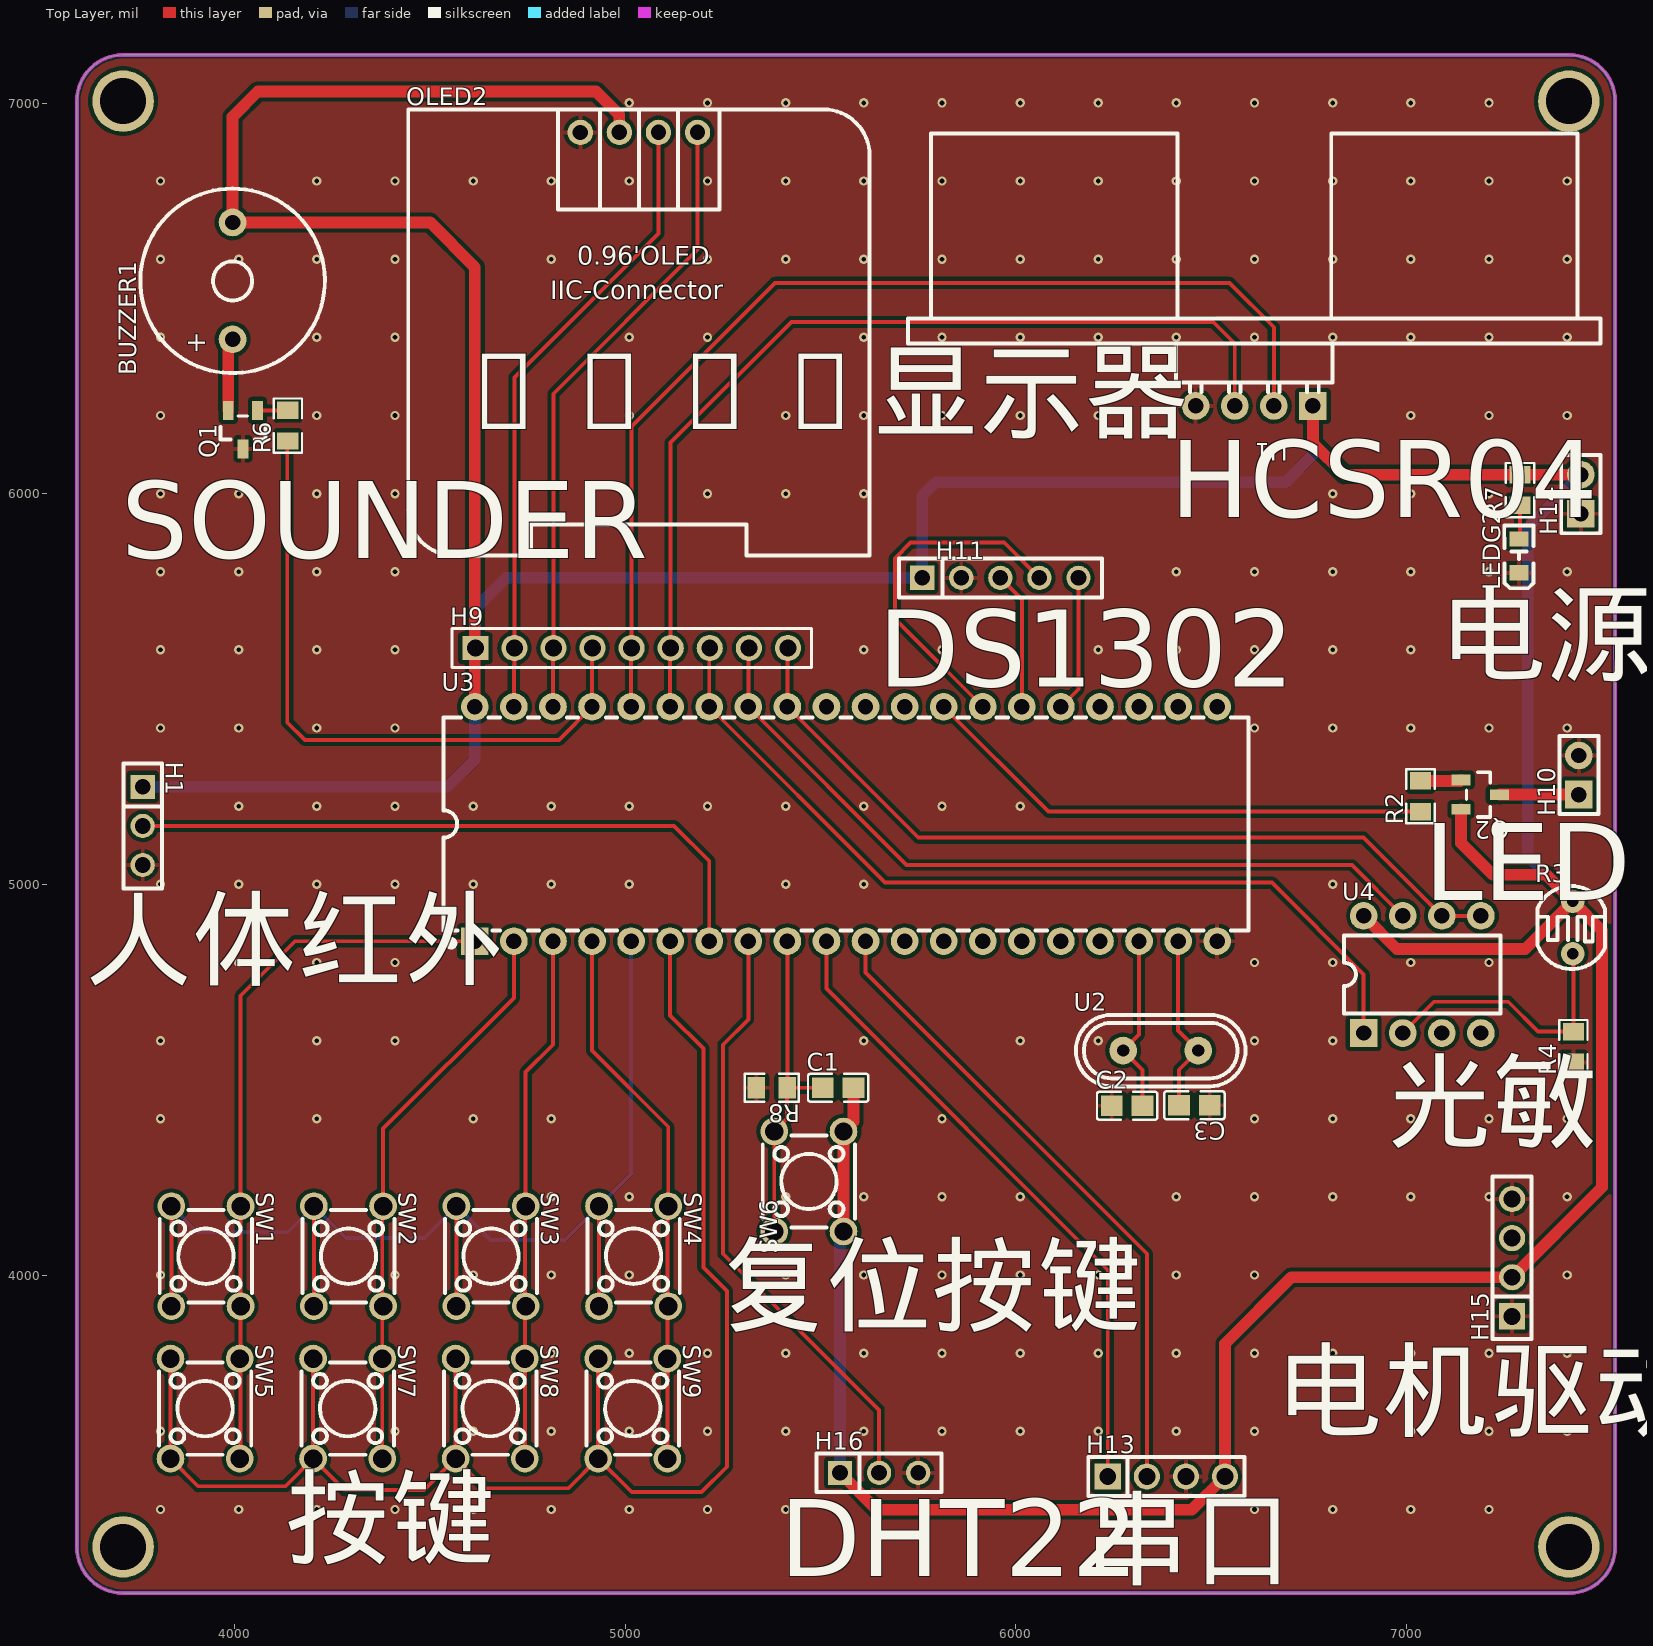
[diagram p0: Top Layer view]
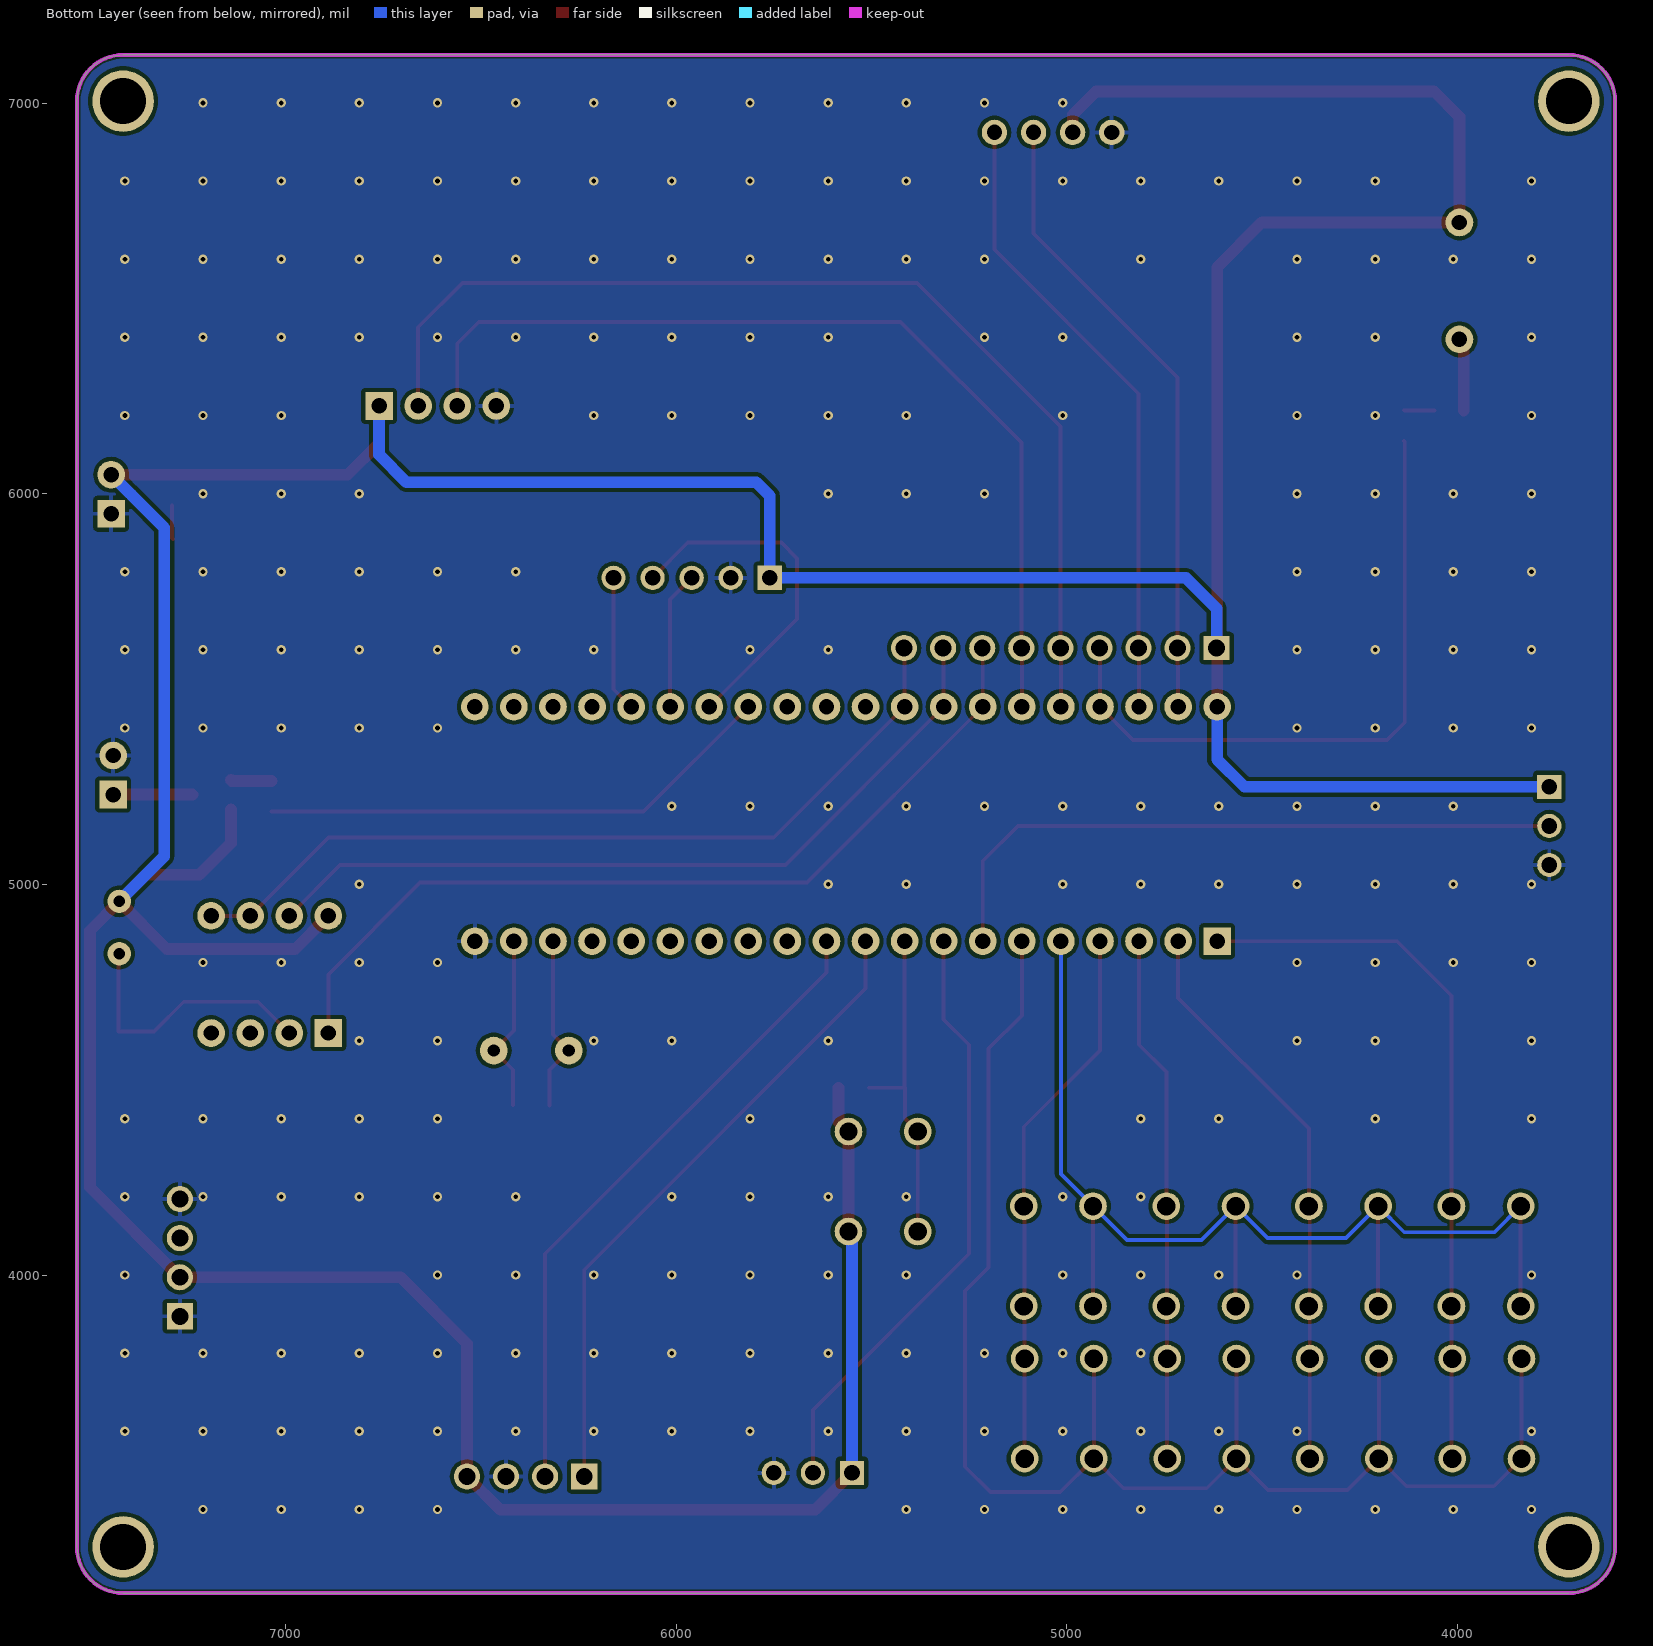
[diagram p1: Bottom Layer view, seen from below]
# Altium PCB MISC52077.pcbdoc
Units mil, origin at the board's own origin, x right, y up, seen from the top; angles counter-clockwise.
Board outline 3937.01 x 3937.01 mil, 2 copper layers (Top Layer, Bottom Layer), stack 62.206 mil thick; 35 components, 34 nets, 158 pads, 232 vias.

## Layer stack, top to bottom
Top Solder Mask Layer: solder mask 0.394, Dk 3.3
Top Layer: signal copper 1.379
Dielectric1: surface 59.449, FR4, Dk 4.5
Bottom Layer: signal copper 1.378
Bottom Solder Mask Layer: solder mask 0.394, Dk 3.3

## Board outline
3596.5,3304.61 ccw(c3714.61,3304.61) 3714.61,3186.5 7415.39,3186.5 ccw(c7415.39,3304.61) 7533.5,3304.61 7533.5,7005.39 ccw(c7415.39,7005.39) 7415.39,7123.5 3714.61,7123.5 ccw(c3714.61,7005.39) 3596.5,7005.39

## Design rules (kind name [scope] priority, off if disabled: settings)
BoardOutlineClearance copperThickness2oz_1 [All] p2 off: genericclearance=7.99 ignorepadtopadclearanceinfootprint=FALSE except(0: Arc-SplitContinuation Track-SplitContinuation SMDPad-SplitContinuation THPad-SplitContinuation Via-SplitContinuation Fill-SplitContinuation Region-SplitContinuation Poly-SplitContinuation Text-SplitContinuation Hole-SplitContinuation; 5.98: Arc-CutoutEdge Track-CutoutEdge SMDPad-CutoutEdge THPad-CutoutEdge Via-CutoutEdge Text-CutoutEdge; 6.9: Hole-OutlineEdge Hole-CutoutEdge; 10: Poly-OutlineEdge Poly-CutoutEdge; 11.81: Arc-OutlineEdge Track-OutlineEdge SMDPad-OutlineEdge THPad-OutlineEdge Via-OutlineEdge Fill-OutlineEdge Region-OutlineEdge Text-OutlineEdge Fill-CutoutEdge Region-CutoutEdge)
BoardOutlineClearance Plane_innerPlane_1 [All] p4 off: genericclearance=4.02 ignorepadtopadclearanceinfootprint=FALSE except(0: Arc-SplitContinuation Track-SplitContinuation SMDPad-SplitContinuation THPad-SplitContinuation Via-SplitContinuation Fill-SplitContinuation Region-SplitContinuation Poly-SplitContinuation Text-SplitContinuation Hole-SplitContinuation; 5.98: Arc-CutoutEdge Track-CutoutEdge SMDPad-CutoutEdge THPad-CutoutEdge Via-CutoutEdge Text-CutoutEdge; 6.9: Hole-OutlineEdge Hole-CutoutEdge; 10: Poly-OutlineEdge Poly-CutoutEdge; 11.81: Arc-OutlineEdge Track-OutlineEdge SMDPad-OutlineEdge THPad-OutlineEdge Via-OutlineEdge Fill-OutlineEdge Region-OutlineEdge Text-OutlineEdge Fill-CutoutEdge Region-CutoutEdge)
BoardOutlineClearance Copper_copperRegion_1 [All] p6 off: genericclearance=4.02 ignorepadtopadclearanceinfootprint=FALSE except(0: Arc-SplitContinuation Track-SplitContinuation SMDPad-SplitContinuation THPad-SplitContinuation Via-SplitContinuation Fill-SplitContinuation Region-SplitContinuation Poly-SplitContinuation Text-SplitContinuation Hole-SplitContinuation; 5.98: Arc-CutoutEdge Track-CutoutEdge SMDPad-CutoutEdge THPad-CutoutEdge Via-CutoutEdge Text-CutoutEdge; 6.9: Hole-OutlineEdge Hole-CutoutEdge; 10: Poly-OutlineEdge Poly-CutoutEdge; 11.81: Arc-OutlineEdge Track-OutlineEdge SMDPad-OutlineEdge THPad-OutlineEdge Via-OutlineEdge Fill-OutlineEdge Region-OutlineEdge Text-OutlineEdge Fill-CutoutEdge Region-CutoutEdge)
BoardOutlineClearance Copper_copperRegion_copperThickness1oz_1 [All] p8 off: genericclearance=4.02 ignorepadtopadclearanceinfootprint=FALSE except(0: Arc-SplitContinuation Track-SplitContinuation SMDPad-SplitContinuation THPad-SplitContinuation Via-SplitContinuation Fill-SplitContinuation Region-SplitContinuation Poly-SplitContinuation Text-SplitContinuation Hole-SplitContinuation; 5.98: Arc-CutoutEdge Track-CutoutEdge SMDPad-CutoutEdge THPad-CutoutEdge Via-CutoutEdge Text-CutoutEdge; 6.9: Hole-OutlineEdge Hole-CutoutEdge; 10: Poly-OutlineEdge Poly-CutoutEdge; 11.81: Arc-OutlineEdge Track-OutlineEdge SMDPad-OutlineEdge THPad-OutlineEdge Via-OutlineEdge Fill-OutlineEdge Region-OutlineEdge Text-OutlineEdge Fill-CutoutEdge Region-CutoutEdge)
BoardOutlineClearance Copper_copperRegion_Copper_copperRegion_1 [All] p10 off: genericclearance=4.02 ignorepadtopadclearanceinfootprint=FALSE except(0: Arc-SplitContinuation Track-SplitContinuation SMDPad-SplitContinuation THPad-SplitContinuation Via-SplitContinuation Fill-SplitContinuation Region-SplitContinuation Poly-SplitContinuation Text-SplitContinuation Hole-SplitContinuation; 5.98: Arc-CutoutEdge Track-CutoutEdge SMDPad-CutoutEdge THPad-CutoutEdge Via-CutoutEdge Text-CutoutEdge; 6.9: Hole-OutlineEdge Hole-CutoutEdge; 10: Poly-OutlineEdge Poly-CutoutEdge; 11.81: Arc-OutlineEdge Track-OutlineEdge SMDPad-OutlineEdge THPad-OutlineEdge Via-OutlineEdge Fill-OutlineEdge Region-OutlineEdge Text-OutlineEdge Fill-CutoutEdge Region-CutoutEdge)
BoardOutlineClearance copperThickness1oz_1 [All] p12: genericclearance=4.02 ignorepadtopadclearanceinfootprint=FALSE except(0: Arc-SplitContinuation Track-SplitContinuation SMDPad-SplitContinuation THPad-SplitContinuation Via-SplitContinuation Fill-SplitContinuation Region-SplitContinuation Poly-SplitContinuation Text-SplitContinuation Hole-SplitContinuation; 5.98: Arc-CutoutEdge Track-CutoutEdge SMDPad-CutoutEdge THPad-CutoutEdge Via-CutoutEdge Text-CutoutEdge; 6.9: Hole-OutlineEdge Hole-CutoutEdge; 10: Poly-OutlineEdge Poly-CutoutEdge; 11.81: Arc-OutlineEdge Track-OutlineEdge SMDPad-OutlineEdge THPad-OutlineEdge Via-OutlineEdge Fill-OutlineEdge Region-OutlineEdge Text-OutlineEdge Fill-CutoutEdge Region-CutoutEdge)
Clearance copperThickness2oz [All] p1 off: gap=7.99 ignorepadtopadclearanceinfootprint=FALSE except(5.98: SMDPad-Track SMDPad-SMDPad THPad-Track SMDPad-THPad THPad-THPad Track-Via SMDPad-Via THPad-Via Via-Via Fill-SMDPad Region-SMDPad Fill-THPad Region-THPad Fill-Via Region-Via Fill-Fill Fill-Region Region-Region Arc-Track Arc-SMDPad Arc-THPad Arc-Via Fill-Arc Region-Arc Arc-Arc Text-Track SMDPad-Text Text-THPad Text-Via Fill-Text Region-Text Arc-Text Text-Text; 6.9: Hole-Track Hole-SMDPad Hole-THPad Hole-Via Fill-Hole Region-Hole Hole-Arc Hole-Text; 10: Poly-Track Poly-SMDPad Poly-THPad Poly-Via Poly-Fill Poly-Region Poly-Poly Poly-Arc Poly-Text Poly-Hole; 11.81: Fill-Track Region-Track)
Clearance Plane_innerPlane [All] p3 off: gap=4.02 ignorepadtopadclearanceinfootprint=FALSE except(5.98: SMDPad-Track SMDPad-SMDPad THPad-Track SMDPad-THPad THPad-THPad Track-Via SMDPad-Via THPad-Via Via-Via Fill-SMDPad Region-SMDPad Fill-THPad Region-THPad Fill-Via Region-Via Fill-Fill Fill-Region Region-Region Arc-Track Arc-SMDPad Arc-THPad Arc-Via Fill-Arc Region-Arc Arc-Arc Text-Track SMDPad-Text Text-THPad Text-Via Fill-Text Region-Text Arc-Text Text-Text; 6.9: Hole-Track Hole-SMDPad Hole-THPad Hole-Via Fill-Hole Region-Hole Hole-Arc Hole-Text; 10: Poly-Track Poly-SMDPad Poly-THPad Poly-Via Poly-Fill Poly-Region Poly-Poly Poly-Arc Poly-Text Poly-Hole; 11.81: Fill-Track Region-Track)
Clearance Copper_copperRegion [All] p5 off: gap=4.02 ignorepadtopadclearanceinfootprint=FALSE except(5.98: SMDPad-Track SMDPad-SMDPad THPad-Track SMDPad-THPad THPad-THPad Track-Via SMDPad-Via THPad-Via Via-Via Fill-SMDPad Region-SMDPad Fill-THPad Region-THPad Fill-Via Region-Via Fill-Fill Fill-Region Region-Region Arc-Track Arc-SMDPad Arc-THPad Arc-Via Fill-Arc Region-Arc Arc-Arc Text-Track SMDPad-Text Text-THPad Text-Via Fill-Text Region-Text Arc-Text Text-Text; 6.9: Hole-Track Hole-SMDPad Hole-THPad Hole-Via Fill-Hole Region-Hole Hole-Arc Hole-Text; 10: Poly-Track Poly-SMDPad Poly-THPad Poly-Via Poly-Fill Poly-Region Poly-Poly Poly-Arc Poly-Text Poly-Hole; 11.81: Fill-Track Region-Track)
Clearance Copper_copperRegion_copperThickness1oz [All] p7 off: gap=4.02 ignorepadtopadclearanceinfootprint=FALSE except(5.98: SMDPad-Track SMDPad-SMDPad THPad-Track SMDPad-THPad THPad-THPad Track-Via SMDPad-Via THPad-Via Via-Via Fill-SMDPad Region-SMDPad Fill-THPad Region-THPad Fill-Via Region-Via Fill-Fill Fill-Region Region-Region Arc-Track Arc-SMDPad Arc-THPad Arc-Via Fill-Arc Region-Arc Arc-Arc Text-Track SMDPad-Text Text-THPad Text-Via Fill-Text Region-Text Arc-Text Text-Text; 6.9: Hole-Track Hole-SMDPad Hole-THPad Hole-Via Fill-Hole Region-Hole Hole-Arc Hole-Text; 10: Poly-Track Poly-SMDPad Poly-THPad Poly-Via Poly-Fill Poly-Region Poly-Poly Poly-Arc Poly-Text Poly-Hole; 11.81: Fill-Track Region-Track)
Clearance Copper_copperRegion_Copper_copperRegion [All] p9 off: gap=4.02 ignorepadtopadclearanceinfootprint=FALSE except(5.98: SMDPad-Track SMDPad-SMDPad THPad-Track SMDPad-THPad THPad-THPad Track-Via SMDPad-Via THPad-Via Via-Via Fill-SMDPad Region-SMDPad Fill-THPad Region-THPad Fill-Via Region-Via Fill-Fill Fill-Region Region-Region Arc-Track Arc-SMDPad Arc-THPad Arc-Via Fill-Arc Region-Arc Arc-Arc Text-Track SMDPad-Text Text-THPad Text-Via Fill-Text Region-Text Arc-Text Text-Text; 6.9: Hole-Track Hole-SMDPad Hole-THPad Hole-Via Fill-Hole Region-Hole Hole-Arc Hole-Text; 10: Poly-Track Poly-SMDPad Poly-THPad Poly-Via Poly-Fill Poly-Region Poly-Poly Poly-Arc Poly-Text Poly-Hole; 11.81: Fill-Track Region-Track)
Clearance copperThickness1oz [All] p11: gap=4.02 ignorepadtopadclearanceinfootprint=FALSE except(5.98: SMDPad-Track SMDPad-SMDPad THPad-Track SMDPad-THPad THPad-THPad Track-Via SMDPad-Via THPad-Via Via-Via Fill-SMDPad Region-SMDPad Fill-THPad Region-THPad Fill-Via Region-Via Fill-Fill Fill-Region Region-Region Arc-Track Arc-SMDPad Arc-THPad Arc-Via Fill-Arc Region-Arc Arc-Arc Text-Track SMDPad-Text Text-THPad Text-Via Fill-Text Region-Text Arc-Text Text-Text; 6.9: Hole-Track Hole-SMDPad Hole-THPad Hole-Via Fill-Hole Region-Hole Hole-Arc Hole-Text; 10: Poly-Track Poly-SMDPad Poly-THPad Poly-Via Poly-Fill Poly-Region Poly-Poly Poly-Arc Poly-Text Poly-Hole; 11.81: Fill-Track Region-Track)
DiffPairsRouting differentialPair [All] p1: maxlimit=6 minlimit=6 mostfreqgap=6 toplayer_minwidth=5 toplayer_prefwidth=10 toplayer_maxwidth=100 toplayer_mingap=6 toplayer_prefgap=6 toplayer_maxgap=6 bottomlayer_minwidth=5 bottomlayer_prefwidth=10 bottomlayer_maxwidth=100 bottomlayer_mingap=6 bottomlayer_prefgap=6 bottomlayer_maxgap=6 maxuncoupledlength=10
HoleToHoleClearance otherClearance [All] p1: gap=11.81 allowstackedmicrovias=TRUE
Length netLength [All] p1: minlimit=0 maxlimit=0
PasteMaskExpansion pasteMaskExpansion [All] p1: expansion=0
PlaneConnect innerPlane [All] p1: planeconnectstyle=Relief reliefexpansion=20 reliefentries=4 reliefconductorwidth=10 reliefairgap=10
PolygonConnect copperRegion_copperThickness1oz [All] p1 off: connectstyle=Relief reliefconductorwidth=10 reliefentries=4 polygonreliefangle="90 Angle" airgapwidth=10 via.connectstyle=Relief via.reliefconductorwidth=10 via.reliefentries=4 via.polygonreliefangle="90 Angle" via.airgapwidth=10
PolygonConnect copperRegion_Copper_copperRegion [All] p2 off: connectstyle=Relief reliefconductorwidth=10 reliefentries=4 polygonreliefangle="90 Angle" airgapwidth=10 via.connectstyle=Relief via.reliefconductorwidth=10 via.reliefentries=4 via.polygonreliefangle="90 Angle" via.airgapwidth=10
PolygonConnect copperRegion [All] p3: connectstyle=Relief reliefconductorwidth=10 reliefentries=4 polygonreliefangle="90 Angle" airgapwidth=10 via.connectstyle=Relief via.reliefconductorwidth=10 via.reliefentries=4 via.polygonreliefangle="90 Angle" via.airgapwidth=10
RoutingVias viaSize [All] p1: holewidth=12.01 width=24.02 viastyle="Through Hole" minholewidth=11.81 minwidth=19.68 maxholewidth=248.03 maxwidth=393.7
SolderMaskExpansion solderMaskExpansion [IsVia] p1: expansion=-1000 istentingtop=TRUE
SolderMaskExpansion solderMaskExpansion [All] p2: expansion=2 istentingtop=FALSE
Width copperThickness2oz_2 [All] p1 off: maxlimit=100 minlimit=8 preferedwidth=10
Width copperThickness1oz_2 [All] p2: maxlimit=100 minlimit=5 preferedwidth=10

## Components (designator, comment, footprint, x,y, rotation, side; value= is the part's Value field where it differs from the comment)
BUZZER1 "buzzer-12X9" BUZ-TH_BD12.0-P7.60-D0.6-FD 3995,6545 r90 top
C1 "10uf" C0805 5545,4480 r0 top
C2 "30pf" C0805 6284.61,4433.87 r0 top
C3 "30pf" C0805 6456.69,4435.13 r180 top
H1 "" HDR-TH_3P-P2.54-V-F 3765,5150 r270 top
H9 "" HDR-TH_9P-P2.54-V-F-1 5016.31,5605.33 r0 top
H10 "" HDR-TH_2P-P2.54-V-M-1 7440.71,5280.33 r90 top
H11 "" HDR-TH_5P-P2.54-V-F 5960,5785 r0 top
H13 "" HDR-TH_4P-P2.54-V-M 6385,3485 r0 top
H14 "" HDR-TH_2P-P2.54-V-M-1 7445.71,5999.16 r90 top
H15 "" HDR-TH_4P-P2.54-V-F 7270,4045 r90 top
H16 "" HDR-TH_3P-P2.54-V-F 5649.7,3494.21 r0 top
LEDG2 "" LED_0805 7287.85,5843.02 r90 top
OLED2 "" 0.96OLED_4P 5035,6925 r0 top
Q1 "2N3906S-RTK/PS" SOT-23-3_L2.9-W1.3-P1.90-LS2.4-TR 4021.38,6164.29 r90 top
Q2 "" S8550P_SOT 7190,5230 r180 top
R2 "1K" R0805 7035.36,5225.96 r90 top
R3 "GL5549(80-100)" RES-TH_L5.1-W4.3-P3.40-D0.5 7425,4890 r0 top
R4 "10K" R0805 7426.63,4584.18 r90 top
R6 "2.2K" R0805 4136.38,6174.61 r90 top
R7 "220" R0805 7290.08,6009.79 r90 top
R8 "10K" R0805 5375,4480 r180 top
SW1 "" SW-TH_4P-L6.0-W6.0-P4.50-LS6.5 3926.76,4048.86 r270 top
SW2 "" SW-TH_4P-L6.0-W6.0-P4.50-LS6.5 4291.63,4048.86 r270 top
SW3 "" SW-TH_4P-L6.0-W6.0-P4.50-LS6.5 4656.5,4048.86 r270 top
SW4 "" SW-TH_4P-L6.0-W6.0-P4.50-LS6.5 5021.37,4048.86 r270 top
SW5 "" SW-TH_4P-L6.0-W6.0-P4.50-LS6.5 3924.68,3658.86 r270 top
SW6 "" SW-TH_4P-L6.0-W6.0-P4.50-LS6.5 5470,4240 r90 top
SW7 "" SW-TH_4P-L6.0-W6.0-P4.50-LS6.5 4289.55,3658.86 r270 top
SW8 "" SW-TH_4P-L6.0-W6.0-P4.50-LS6.5 4654.42,3658.86 r270 top
SW9 "" SW-TH_4P-L6.0-W6.0-P4.50-LS6.5 5019.29,3658.86 r270 top
U1 "HC-SR04" TH_HC-SR04V 6610,6225 r180 top
U2 "11.0592MHz" HC-49US_L11.0-W4.6-P4.88 6370.43,4575.13 r0 top
U3 "STC89C516RD+40I-PDIP40" DIP-40_L52.3-W13.9-P2.54-LS15.2-BL 5565,5155 r0 top
U4 "ADC0832CCN" DIP-8_L9.7-W6.4-P2.54-LS7.6-BL 7040,4770 r0 top

## Footprints (in the part's own frame and the unit in brackets; to place one, negate y for a bottom-side part, rotate by r counter-clockwise, add the part's x,y. Pads: shape width x height; smd on the part's side, far side on the other; paste and mask are expansions set on the pad)
0.96OLED_4P [mm]
  round 1.65 hole 1 copper offset 0,0: 1(-3.81,-0.001) 2(-1.27,0.002) 3(1.27,0.002) 4(3.81,0.002)
  silkscreen extent -15,-27.5 15,1.5
BUZ-TH_BD12.0-P7.60-D0.6-FD [mm]
  round 1.8 hole 1: 1(-3.8,0) 2(3.8,0)
  silkscreen extent -6,-6 6,6
C0805 [mm]
  rect 1.41x1.35 smd paste-100 mask+0.051: 1(-1,0) 2(1,0)
  silkscreen extent -1.96,-0.9 1.96,0.9
DIP-8_L9.7-W6.4-P2.54-LS7.6-BL [mm]
  rect 1.8x1.8 hole 1 paste+0 mask+0.05: 1(-3.81,-3.81)
  round 1.8 hole 1 paste+0 mask+0.05: 2(-1.27,-3.81) 3(1.27,-3.81) 4(3.81,-3.81) 5(3.81,3.81) 6(1.27,3.81) 7(-1.27,3.81) 8(-3.81,3.81)
  silkscreen extent -5.08,-2.53 5.08,2.53
DIP-40_L52.3-W13.9-P2.54-LS15.2-BL [mm]
  rect 1.8x1.8 hole 1: 1(-24.13,-7.62)
  round 1.8 hole 1: 2(-21.59,-7.62) 3(-19.05,-7.62) 4(-16.51,-7.62) 5(-13.97,-7.62) 6(-11.43,-7.62) 7(-8.89,-7.62) 8(-6.35,-7.62) 9(-3.81,-7.62) 10(-1.27,-7.62) 11(1.27,-7.62) 12(3.81,-7.62) 13(6.35,-7.62) 14(8.89,-7.62) 15(11.43,-7.62) 16(13.97,-7.62) 17(16.51,-7.62) 18(19.05,-7.62) 19(21.59,-7.62) 20(24.13,-7.62) 21(24.13,7.62) 22(21.59,7.62) 23(19.05,7.62) 24(16.51,7.62) 25(13.97,7.62) 26(11.43,7.62) 27(8.89,7.62) 28(6.35,7.62) 29(3.81,7.62) 30(1.27,7.62) 31(-1.27,7.62) 32(-3.81,7.62) 33(-6.35,7.62) 34(-8.89,7.62) 35(-11.43,7.62) 36(-13.97,7.62) 37(-16.51,7.62) 38(-19.05,7.62) 39(-21.59,7.62) 40(-24.13,7.62)
  silkscreen extent -26.16,-7.95 26.16,6.93
HC-49US_L11.0-W4.6-P4.88 [mm]
  round 1.8 hole 0.8: 1(-2.44,0) 2(2.44,0)
  silkscreen extent -5.51,-2.32 5.51,2.32
HDR-TH_2P-P2.54-V-M-1 [mm]
  rect 1.8x1.8 hole 1: 1(-1.27,0)
  round 1.8 hole 1: 2(1.27,0)
  silkscreen extent -2.54,-1.27 2.54,1.27
HDR-TH_3P-P2.54-V-F [mil]
  rect 62x62 hole 40.16: 1(-100,0)
  round 62 hole 40.16: 2(0,0) 3(100,0)
  silkscreen extent -160,-49 160,49
HDR-TH_4P-P2.54-V-F [mm]
  rect 1.7x1.7 hole 1.1: 1(-3.81,0)
  round 1.7 hole 1.1: 2(-1.27,0) 3(1.27,0) 4(3.81,0)
  silkscreen extent -5.29,-1.27 5.29,1.27
HDR-TH_4P-P2.54-V-M [mm]
  rect 1.7x1.7 hole 1.1: 1(-3.81,0)
  round 1.7 hole 1.1: 2(-1.27,0) 3(1.27,0) 4(3.81,0)
  silkscreen extent -5.08,-1.27 5.08,1.27
HDR-TH_5P-P2.54-V-F [mil]
  rect 62x62 hole 40.16: 1(-200,0)
  round 62 hole 40.16: 2(-100,0) 3(0,0) 4(100,0) 5(200,0)
  silkscreen extent -260,-50 260,50
HDR-TH_9P-P2.54-V-F-1 [mm]
  rect 1.7x1.575 hole 1.1: 1(-10.16,0)
  round 1.7 hole 1.1: 2(-7.62,0) 3(-5.08,0) 4(-2.54,0) 5(0,0) 6(2.54,0) 7(5.08,0) 8(7.62,0) 9(10.16,0)
  silkscreen extent -11.68,-1.27 11.68,1.27
LED_0805 [mm]
  rect 1x1.25 smd paste+0 mask+0.051: 1(-1.15,0.005) 2(1.05,0.005)
  silkscreen extent -2.15,-0.94 1.93,0.97
R0805 [mm]
  rect 1.133x1.377 smd paste-100 mask+0.051: 1(-1,0) 2(1,0)
  silkscreen extent -1.76,-0.92 1.76,0.92
RES-TH_L5.1-W4.3-P3.40-D0.5 [mil]
  round 60 hole 30: 1(0,66.93) 2(0,-66.93)
  silkscreen extent -91,-106 83,106
S8550P_SOT [mil]
  rect 49.2x27.6 smd paste+0 mask+2: 1(50.84,-37.4) 2(50.84,37.4) 3(-47.56,0)
  silkscreen extent -24,-58 37,58
SOT-23-3_L2.9-W1.3-P1.90-LS2.4-TR [mm]
  rect 1.25x0.7 smd: 1(1.25,0.95) 2(1.25,-0.95) 3(-1.25,0)
  silkscreen extent -0.65,-1.46 0.9,1.46
SW-TH_4P-L6.0-W6.0-P4.50-LS6.5 [mm]
  round 1.8 hole 1.2: 1(-3.25,2.25) 2(3.25,2.25) 3(-3.25,-2.25) 4(3.25,-2.25)
  silkscreen extent -3,-3 3,3
TH_HC-SR04V [mm]
  rect 1.8x1.8 hole 1.001: 1(-3.81,0)
  round 1.8 hole 1.001: 2(-1.27,0) 3(1.27,0) 4(3.81,0)
  silkscreen extent -22.5,-17.7 22.5,-0.89

## Free pads (board coordinates)
  round 157.48 hole 118.11: 1(3714.61,7005.39) 1(3714.61,3304.61) 1(7415.39,7005.39) 1(7415.39,3304.61)

## Via types
v1: diameter 24.02, hole 12, Top Layer to Bottom Layer, 232 vias

## Nets (pads, with @x,y where several pads share a name; then routed paths per layer and width w, separated by ;. In a path a pad name is that pad's centre, name@x,y a point inside that pad or via, vN(x,y) a via of type N, cw(c..) or ccw(c..) an arc to the next point about the centre after c; other vN are vias at no path point)
$1N17166: LEDG2.2 R7.1 | length 87.1
  Top Layer w10: LEDG2.2 7290.08,5886.8 R7.1
$1N17180: C1.1 R8.1 SW6.1 SW6.2 U3.9 | length 848.1
  Top Layer w10: SW6.1 5381.42,4367.95 5414.37,4400.9 R8.1 ; U3.9 5415,4480.63 R8.1 ; C1.1 R8.1
$1N17214: C3.2 U2.2 U3.19 | length 461.6
  Top Layer w10: U3.19 6415,4626.62 U2.2 6417.32,4525.96 C3.2
$1N17215: C2.2 U2.1 U3.18 | length 458.5
  Top Layer w10: U3.18 6315,4615.76 U2.1 6323.98,4525.52 C2.2
$1N17240: BUZZER1.1 Q1.1 | length 186.5
  Top Layer w30: Q1.1 3983.98,6384.37 BUZZER1.1
$1N17242: Q1.2 R6.2 | length 77.8
  Top Layer w10: Q1.2 4135.89,6213.49 R6.2
$1N17247: R2.1 U3.28 | length 1331.5
  Top Layer w10: U3.28 6083.41,5186.59 R2.1
$1N17248: Q2.1 R2.2 | length 104.7
  Top Layer w30: R2.2 7137.09,5265.33 Q2.1
$1N17250: H10.1 Q2.3 | length 203.3
  Top Layer w30: Q2.3 7237.89,5230.33 H10.1
$1N17273: R3.2 R4.2 U4.2 | length 701.6
  Top Layer w10: U4.2 7070,4700 7260,4700 7336.45,4623.55 R4.2 7426.63,4821.44 R3.2
$1N17284: H16.2 U3.8 | length 1553.3
  Top Layer w10: U3.8 5315,4655 5250,4590 5250,4055 5649.7,3655.3 H16.2
$1N17289: H1.2 U3.7 | length 1692.3
  Top Layer w10: H1.2 5125,5150 5215,5060 U3.7
EC: H9.6 U1.3 U3.35 | length 2431.2
  Top Layer w10: U3.35 5115,5604.02 H9.6 5116.31,6131.31 5425,6440 6505,6440 6560,6385 U1.3
GND: C2.1 C3.1 H1.3 H10.2 H11.2 H13.3 H14.1 H15.1 H15.4 H16.3 LEDG2.1 OLED2.1 Q1.3 R4.1 R8.2 U1.4 U3.20
  other v1: 3810.6,3400.6 4010.6,3400.6 4210.6,3400.6 4410.6,3400.6 4610.6,3400.6 4810.6,3400.6 5010.6,3400.6 5210.6,3400.6 5410.6,3400.6 6610.6,3400.6 6810.6,3400.6 7010.6,3400.6 7210.6,3400.6 3810.6,3600.6 4410.6,3600.6 4610.6,3600.6 4810.6,3600.6 5010.6,3600.6 5210.6,3600.6 5410.6,3600.6 5610.6,3600.6 5810.6,3600.6 6010.6,3600.6 6210.6,3600.6 6410.6,3600.6 6610.6,3600.6 6810.6,3600.6 7010.6,3600.6 7210.6,3600.6 7410.6,3600.6 4810.6,3800.6 5010.6,3800.6 5210.6,3800.6 5410.6,3800.6 5610.6,3800.6 5810.6,3800.6 6010.6,3800.6 6210.6,3800.6 6410.6,3800.6 6610.6,3800.6 6810.6,3800.6 7010.6,3800.6 7210.6,3800.6 7410.6,3800.6 3810.6,4000.6 4410.6,4000.6 4610.6,4000.6 4810.6,4000.6 5010.6,4000.6 5410.6,4000.6 5610.6,4000.6 5810.6,4000.6 6010.6,4000.6 6210.6,4000.6 6410.6,4000.6 6610.6,4000.6 7410.6,4000.6 4810.6,4200.6 5010.6,4200.6 5410.6,4200.6 5610.6,4200.6 5810.6,4200.6 6010.6,4200.6 6410.6,4200.6 6610.6,4200.6 6810.6,4200.6 7010.6,4200.6 7210.6,4200.6 7410.6,4200.6 3810.6,4400.6 4210.6,4400.6 4610.6,4400.6 4810.6,4400.6 5810.6,4400.6 6610.6,4400.6 6810.6,4400.6 7010.6,4400.6 7210.6,4400.6 7410.6,4400.6 3810.6,4600.6 4210.6,4600.6 4410.6,4600.6 5610.6,4600.6 6010.6,4600.6 6210.6,4600.6 6610.6,4600.6 6810.6,4600.6 3810.6,4800.6 4010.6,4800.6 4210.6,4800.6 4410.6,4800.6 6610.6,4800.6 6810.6,4800.6 7010.6,4800.6 7210.6,4800.6 3810.6,5000.6 4010.6,5000.6 4210.6,5000.6 4410.6,5000.6 4610.6,5000.6 4810.6,5000.6 5010.6,5000.6 5410.6,5000.6 5610.6,5000.6 6810.6,5000.6 4010.6,5200.6 4210.6,5200.6 4410.6,5200.6 4610.6,5200.6 4810.6,5200.6 5010.6,5200.6 5210.6,5200.6 5410.6,5200.6 5610.6,5200.6 5810.6,5200.6 6010.6,5200.6 3810.6,5400.6 4010.6,5400.6 4210.6,5400.6 4410.6,5400.6 6610.6,5400.6 6810.6,5400.6 7010.6,5400.6 7210.6,5400.6 7410.6,5400.6 3810.6,5600.6 4010.6,5600.6 4210.6,5600.6 4410.6,5600.6 5610.6,5600.6 5810.6,5600.6 6210.6,5600.6 6410.6,5600.6 6610.6,5600.6 6810.6,5600.6 7010.6,5600.6 7210.6,5600.6 7410.6,5600.6 3810.6,5800.6 4010.6,5800.6 4210.6,5800.6 4410.6,5800.6 6410.6,5800.6 6610.6,5800.6 6810.6,5800.6 7010.6,5800.6 7210.6,5800.6 7410.6,5800.6 3810.6,6000.6 4010.6,6000.6 4210.6,6000.6 4410.6,6000.6 5210.6,6000.6 5410.6,6000.6 5610.6,6000.6 6810.6,6000.6 7010.6,6000.6 7210.6,6000.6 3810.6,6200.6 4210.6,6200.6 4410.6,6200.6 5010.6,6200.6 5410.6,6200.6 5610.6,6200.6 5810.6,6200.6 6010.6,6200.6 6210.6,6200.6 7010.6,6200.6 7210.6,6200.6 7410.6,6200.6 3810.6,6400.6 4210.6,6400.6 4410.6,6400.6 5010.6,6400.6 5210.6,6400.6 5610.6,6400.6 5810.6,6400.6 6010.6,6400.6 6210.6,6400.6 6410.6,6400.6 6610.6,6400.6 6810.6,6400.6 7010.6,6400.6 7210.6,6400.6 7410.6,6400.6 3810.6,6600.6 4010.6,6600.6 4210.6,6600.6 4410.6,6600.6 4810.6,6600.6 5210.6,6600.6 5410.6,6600.6 5610.6,6600.6 5810.6,6600.6 6010.6,6600.6 6210.6,6600.6 6410.6,6600.6 6610.6,6600.6 6810.6,6600.6 7010.6,6600.6 7210.6,6600.6 7410.6,6600.6 3810.6,6800.6 4210.6,6800.6 4410.6,6800.6 4610.6,6800.6 4810.6,6800.6 5010.6,6800.6 5210.6,6800.6 5410.6,6800.6 5610.6,6800.6 5810.6,6800.6 6010.6,6800.6 6210.6,6800.6 6410.6,6800.6 6610.6,6800.6 6810.6,6800.6 7010.6,6800.6 7210.6,6800.6 7410.6,6800.6 5010.6,7000.6 5210.6,7000.6 5410.6,7000.6 5610.6,7000.6 5810.6,7000.6 6010.6,7000.6 6210.6,7000.6 6410.6,7000.6 6610.6,7000.6 6810.6,7000.6 7010.6,7000.6 7210.6,7000.6
P02: H9.4 R6.1 U3.37 | length 1705.5
  Top Layer w10: R6.1 4135,6133.86 4135,5415 4180,5370 4830,5370 U3.37 4915,5604.02 H9.4
P05: H9.7 U3.34 U4.1 | length 2259.6
  Top Layer w10: H9.7 5215,5604.02 U3.34 5665,5005 6655,5005 6890,4770 U4.1
P06: H9.8 U3.33 U4.7 | length 2047.5
  Top Layer w10: H9.8 5315,5604.02 U3.33 5720,5050 6860,5050 U4.7
P07: H9.9 U3.32 U4.5 U4.6 | length 2147.5
  Top Layer w10: H9.9 5415,5604.02 U3.32 5750,5120 6890,5120 U4.6 U4.5
P10: SW1.1 SW1.2 SW5.1 SW5.2 U3.1 | length 1842.8
  Top Layer w10: SW5.2 4015.34,3532.99 SW1.2 SW1.1 4015.34,4715.34 4155,4855 U3.1
P11: SW2.1 SW2.2 SW7.1 SW7.2 U3.2 | length 1463.6
  Top Layer w10: SW7.2 SW7.1 4378.13,4174.72 SW2.1 4380.21,4375.21 4715,4710 U3.2
P12: SW3.1 SW3.2 SW8.1 SW8.2 U3.3 | length 1353.9
  Top Layer w10: SW8.2 SW8.1 4743,4174.72 SW3.1 4745.08,4520.08 4815,4590 U3.3
P13: SW4.1 SW4.2 SW9.1 SW9.2 U3.4 | length 1405.7
  Top Layer w10: U3.4 4915,4575 5109.95,4380.05 SW4.1 5107.87,4174.72 SW9.1 SW9.2
P14: SW1.3 SW1.4 SW2.3 SW2.4 SW3.3 SW3.4 SW4.3 SW4.4 U3.5 | length 3025.5
  Top Layer w10: SW1.4 SW1.3 ; SW2.4 SW2.3 ; SW3.4 SW3.3 ; SW4.4 SW4.3
  Bottom Layer w10: SW1.3 3904.98,4110 4136.24,4110 SW2.3 4284.85,4095 4486.12,4095 SW3.3 4654.73,4090 4845.99,4090 SW4.3 5015,4259.01 U3.5
P15: SW5.3 SW5.4 SW7.3 SW7.4 SW8.3 SW8.4 SW9.3 SW9.4 U3.6 | length 4103.7
  Top Layer w10: SW5.3 SW5.4 3907,3460 4130.06,3460 SW7.4 ; SW7.3 SW7.4 ; SW8.3 SW8.4 ; SW9.3 SW9.4 ; U3.6 5115,4665 5200,4580 5200,4020 5260,3960 5260,3510 5195,3445 5016.62,3445 SW9.4 ; SW7.4 4281.87,3450 4484.93,3450 SW8.4 ; SW8.4 4641.75,3455 4854.81,3455 SW9.4
P24: H11.5 U3.25 | length 348.6
  Top Layer w10: U3.25 6160,5500 H11.5
P25: H11.3 U3.26 | length 352.8
  Top Layer w10: H11.3 6015,5730 U3.26
P26: H11.4 U3.27 | length 897
  Top Layer w10: U3.27 5690,5680 5690,5835 5730,5875 5970,5875 H11.4
P32: H15.3
RX0: H13.1 U3.10 | length 1668.2
  Top Layer w10: U3.10 5515,4733.58 6235,4013.58 H13.1
SCL: H9.2 OLED2.3 U3.39 | length 1623.3
  Top Layer w10: U3.39 4715,5560.55 4716.31,5561.86 H9.2 4716.31,6297.73 5085,6666.42 OLED2.3@5085,6925.05
SDA: H9.3 OLED2.4 U3.38 | length 1623.3
  Top Layer w10: U3.38 4815,5604.02 H9.3 4816.31,6256.31 5185,6625 OLED2.4@5185,6925.05
TR: H9.5 U1.2 U3.36 | length 2762.6
  Top Layer w10: U3.36 5015,5604.02 H9.5 5016.31,6172.73 5383.58,6540 6546.42,6540 6660,6426.42 U1.2
TX0: H13.2 U3.11 | length 1668.2
  Top Layer w10: U3.11 5615,4775 6335,4055 H13.2
VCC: BUZZER1.2 C1.2 H1.1 H9.1 H11.1 H13.4 H14.2 H15.2 H16.1 OLED2.2 Q2.2 R3.1 R7.2 SW6.3 SW6.4 U1.1 U3.40 U4.8 | length 14178
  Top Layer w30: U3.40 4615,6580 4500.4,6694.6 BUZZER1.2 3995,6965 4060,7030 4925,7030 4985,6970 OLED2.2@4985,6925.05 ; H16.1 5643.92,3400 6450,3400 H13.4 6535,3825 6705,3995 H15.2 7500,4225 7500,4881.93 R3.1 ; SW6.3 5558.58,4367.95 5584.37,4393.74 C1.2 ; U1.1 6760,6130 6840.84,6049.16 R7.2 H14.2 ; U4.8 6975,4835 7303.07,4835 R3.1 ; Q2.2 7139.16,5105.84 7220,5025 7356.93,5025 R3.1
  Bottom Layer w30: H1.1 4545,5250 4615,5320 U3.40 ; H9.1 4616.31,5706.31 4695,5785 H11.1 5760,5995 5795,6030 6690,6030 6760,6100 U1.1 ; H16.1 5549.7,4103.17 SW6.3 ; R3.1 7310,5071.93 7310,5913.45 7392.89,5996.34 cw(c7410.28,5984.59) 7398.53,6001.98 H14.2
pads on no net: U3.12 U3.13 U3.14 U3.15 U3.16 U3.17 U3.21 U3.22 U3.23 U3.24 U3.29 U3.30 U3.31 U4.3 U4.4

## Polygon pours and split planes (outlines as drawn)
GND on Bottom Layer (solid, remove dead copper, pour order 2): 3525,7245 3525,3080 7700,3080 7700,7245
GND on Top Layer (solid, remove dead copper, pour order 2): 3000,7415 3000,3000 7930,3000 7930,7415

## Keep-outs
Board Outline Layer:
  the board outline again, w10

## Silkscreen, mask and mechanical layers (free items; w line width, h text height)
Top Silkscreen Layer:
  text "Oled显示器" at 4555,6165 h196.85
  text "HCSR04" at 6395,5940 h196.85
  text "SOUNDER" at 3710,5835 h196.85
  text "电源" at 7090,5545 h196.85
  text "DS1302" at 5647.87,5506.57 h196.85
  text "LED" at 7045,4960 h196.85
  text "人体红外" at 3620,4765 h196.85
  text "光敏" at 6950,4350 h196.85
  text "复位按键" at 5245,3880 h196.85
  text "电机驱动" at 6670,3610 h196.85
  text "按键" at 4130,3285 h196.85
  text "DHT22" at 5395,3230 h196.85
  text "串口" at 6175,3230 h196.85